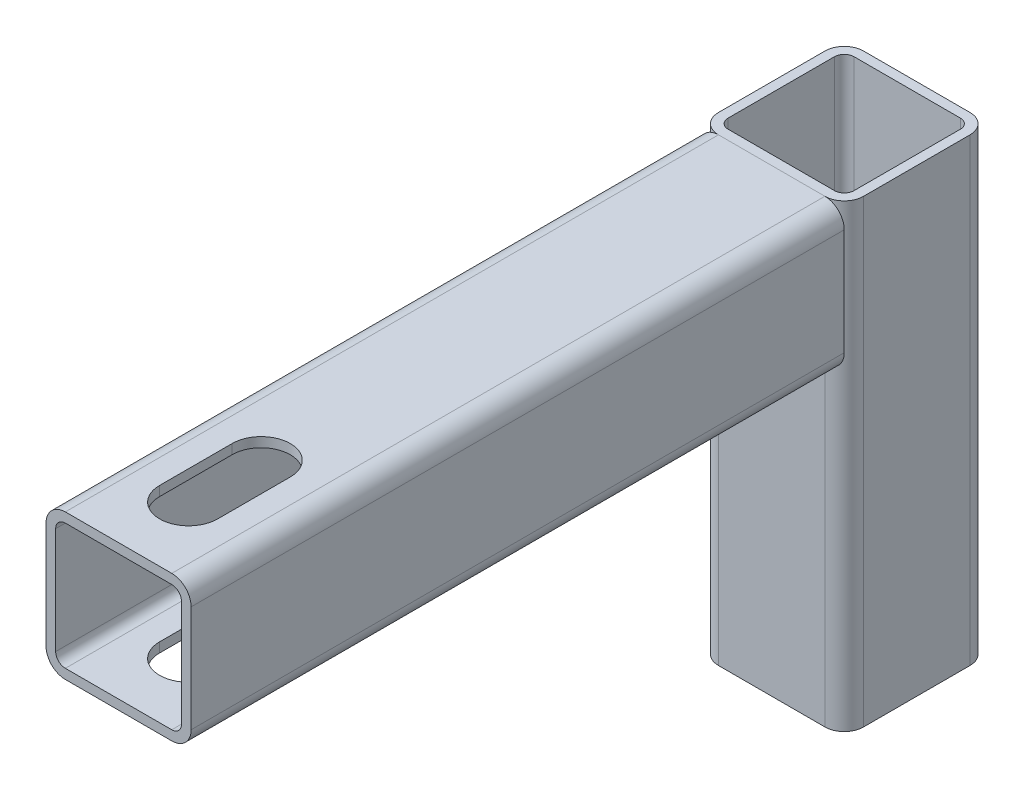
SolidWorks part; units mm, degrees
ref_plane "前视基准面" through (0, 0, 0) normal (0, 0, 1) x (1, 0, 0)
ref_plane "上视基准面" through (0, 0, 0) normal (0, 1, 0) x (1, 0, 0)
ref_plane "右视基准面" through (0, 0, 0) normal (1, 0, 0) x (0, 0, -1)
sketch "草图1" plane through (0, 0, 0) normal (1, 0, 0) x (0, 0, -1)
  line L0 (0, 0) -> (0, 80)
  line L1 (0, 44) -> (0, -44) construction
  line L2 (0, 80) -> (-150, 80)
  dimension "D1" = 80
  dimension "D2" = 150
other "Gb／6728-1986方形空心型钢 030 X 30 X 2(1)"
ref_plane "基准面1" through (0, 80, 0) normal (0, 0, 1) x (0, -1, 0)
sketch "Sketch13" plane through (0, 80, 0) normal (0, 0, 1) x (0, -1, 0)
  line L0 (-11, -13) -> (11, -13)
  line L1 (-13, -11) -> (-13, 11)
  line L2 (11, 13) -> (-11, 13)
  line L3 (13, 11) -> (13, -11)
  line L4 (-11, -15) -> (11, -15)
  line L5 (-15, -11) -> (-15, 11)
  line L6 (11, 15) -> (-11, 15)
  line L7 (15, 11) -> (15, -11)
  arc A0 (15, 11) -> (11, 15) centre (11, 11) ccw
  arc A1 (11, -15) -> (15, -11) centre (11, -11) ccw
  arc A2 (-15, -11) -> (-11, -15) centre (-11, -11) ccw
  arc A3 (-11, 15) -> (-15, 11) centre (-11, 11) ccw
  arc A4 (-11, 13) -> (-13, 11) centre (-11, 11) ccw
  arc A5 (13, 11) -> (11, 13) centre (11, 11) ccw
  arc A6 (11, -13) -> (13, -11) centre (11, -11) ccw
  arc A7 (-13, -11) -> (-11, -13) centre (-11, -11) ccw
  point P0 (-15, 0)
  point P1 (15, 0)
  point P2 (0, 15)
  point P3 (0, -15)
  point P4 (0, 0)
  point P5 (-15, -15)
  point P6 (15, -15)
  point P7 (15, 15)
  point P8 (-15, 15)
  point P33 (0, 0)
  dimension "D1" = 4
  dimension "Thickness" = 2
  dimension "V_leg" = 30
sketch "草图6" plane through (0, 95, 0) normal (0, 1, 0) x (1, 0, 0)
  line L0 (0, -135.5142) -> (0, -120.5142) construction
  line L1 (0, 0) -> (0, -150) construction
  line L2 (-6, -135.5142) -> (-6, -120.5142)
  line L3 (6, -135.5142) -> (6, -120.5142)
  arc A0 (-6, -135.5142) -> (6, -135.5142) centre (0, -135.5142) ccw
  arc A1 (6, -120.5142) -> (-6, -120.5142) centre (0, -120.5142) ccw
  point P4 (0, -128.0142)
  dimension "D1" = 12
  dimension "D2" = 15
extrude "切除-拉伸1" cut sketch "草图6" against normal blind 67
